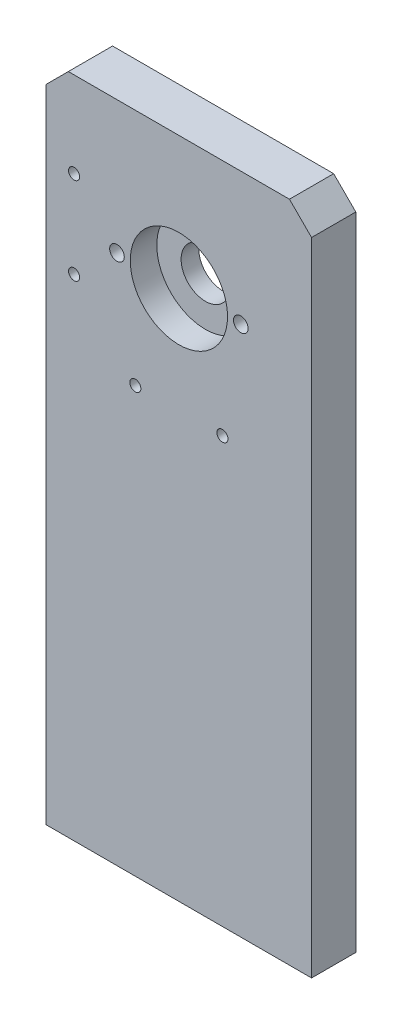
from build123d import *

# Parameters (mm, degrees)
SKETCH1_W             = 60
SKETCH1_H             = 150
BOSS_EXTRUDE1_DEPTH   = 10
CHAMFER1_SIZE         = 5
SKETCH2_R             = 11
CUT_EXTRUDE1_DEPTH    = 6
SKETCH3_R             = 5.5
CUT_EXTRUDE2_DEPTH    = 82
M4_TAPPED_HOLE1_D     = 3.3
M4_TAPPED_HOLE2_D     = 3.3
M4_TAPPED_HOLE2_DEPTH = 11.5
M4_TAPPED_HOLE2_TIP   = 0.991420021
M3_TAPPED_HOLE1_D     = 2.5


with BuildPart() as part:
    # Sketch1 → Boss-Extrude1 (new body)
    with BuildSketch(Plane.XY):
        Rectangle(SKETCH1_W, SKETCH1_H)
    extrude(amount=BOSS_EXTRUDE1_DEPTH)

    # Chamfer1
    chamfer1_edges = [part.edges().sort_by_distance(p)[0] for p in [
        (-30, 75, 5),
        (30, 75, 5),
    ]]
    chamfer(chamfer1_edges, length=CHAMFER1_SIZE)

    # Sketch2 → Cut-Extrude1 (cut)
    with BuildSketch(Plane.XY.offset(10)):
        with Locations((0, 45)):
            Circle(SKETCH2_R)
    extrude(amount=-CUT_EXTRUDE1_DEPTH, mode=Mode.SUBTRACT)

    # Sketch3 → Cut-Extrude2 (cut, through all)
    with BuildSketch(Plane.XY.offset(4)):
        with Locations((0, 45)):
            Circle(SKETCH3_R)
    extrude(amount=-CUT_EXTRUDE2_DEPTH, mode=Mode.SUBTRACT)

    # M4 Tapped Hole1 (through all)
    with Locations(Plane.XY.offset(10)):
        with Locations((-14, 45), (14, 45)):
            Hole(M4_TAPPED_HOLE1_D / 2)

    # M4 Tapped Hole2
    with Locations(Plane(origin=(0, -75, 0), x_dir=(-1, 0, 0), z_dir=(0, -1, 0))):
        with Locations((20, -5), (-20, -5)):
            Hole(M4_TAPPED_HOLE2_D / 2, depth=M4_TAPPED_HOLE2_DEPTH)
            with Locations((0, 0, -(M4_TAPPED_HOLE2_DEPTH + M4_TAPPED_HOLE2_TIP / 2))):  # 118° drill point
                Cone(0, M4_TAPPED_HOLE2_D / 2, M4_TAPPED_HOLE2_TIP, mode=Mode.SUBTRACT)

    # M3 Tapped Hole1 (through all)
    with Locations(Plane(origin=(0, 0, 0), x_dir=(-1, 0, 0), z_dir=(0, 0, -1))):
        with Locations((-9.85, 21.1), (9.85, 21.1), (23.7, 35.95), (23.7, 55.65)):
            Hole(M3_TAPPED_HOLE1_D / 2)


solid = part.part
